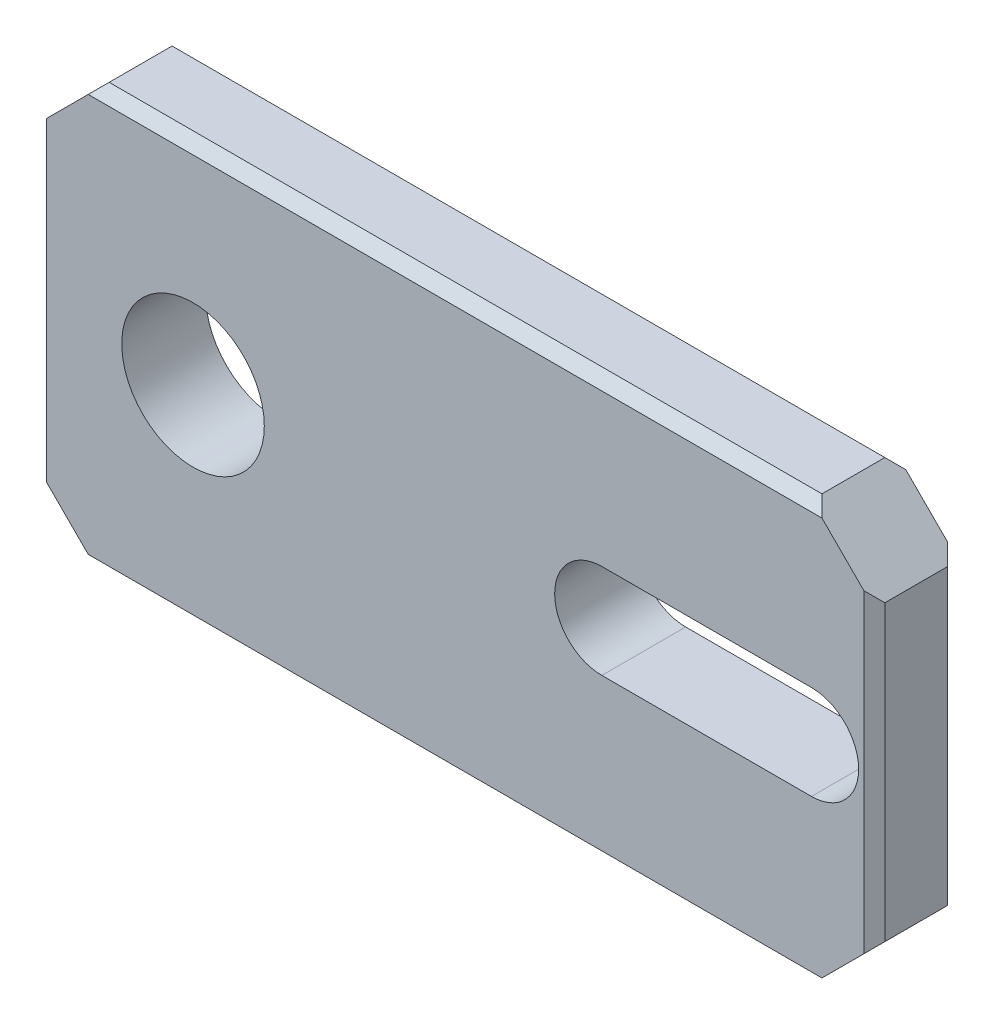
from build123d import *

# Parameters (mm, degrees)
SKETCH1_W           = 40
SKETCH1_H           = 20
BOSS_EXTRUDE1_DEPTH = 4
M8_TAPPED_HOLE1_D   = 6.8
CUT_EXTRUDE1_DEPTH  = 4
CHAMFER1_SIZE       = 3
CHAMFER2_SIZE       = 0.5


with BuildPart() as part:
    # Sketch1 → Boss-Extrude1 (new body)
    with BuildSketch(Plane.XY):
        Rectangle(SKETCH1_W, SKETCH1_H)
    extrude(amount=BOSS_EXTRUDE1_DEPTH)

    # M8 Tapped Hole1 (through all)
    with Locations(Plane.XY.offset(4)):
        with Locations((-12.5, 0)):
            Hole(M8_TAPPED_HOLE1_D / 2)

    # Sketch4 → Cut-Extrude1 (cut)
    with BuildSketch(Plane.XY.offset(4)):
        with BuildLine():
            Line((7, 2.25), (17, 2.25))
            ThreePointArc((17, 2.25), (19.25, 0), (17, -2.25))
            Line((17, -2.25), (7, -2.25))
            ThreePointArc((7, -2.25), (4.75, 0), (7, 2.25))
        make_face()
    extrude(amount=-CUT_EXTRUDE1_DEPTH, mode=Mode.SUBTRACT)

    # Chamfer1
    chamfer1_edges = [part.edges().sort_by_distance(p)[0] for p in [
        (20, -10, 2),
        (-20, -10, 2),
        (-20, 10, 2),
        (20, 10, 2),
    ]]
    chamfer(chamfer1_edges, length=CHAMFER1_SIZE)

    # Chamfer2
    chamfer2_edges = [part.edges().sort_by_distance(p)[0] for p in [
        (20, 0, 0),
        (20, 0, 4),
        (0, -10, 0),
        (-20, 0, 0),
        (0, 10, 0),
        (0, -10, 4),
        (0, 10, 4),
        (-20, 0, 4),
    ]]
    chamfer(chamfer2_edges, length=CHAMFER2_SIZE)


solid = part.part
